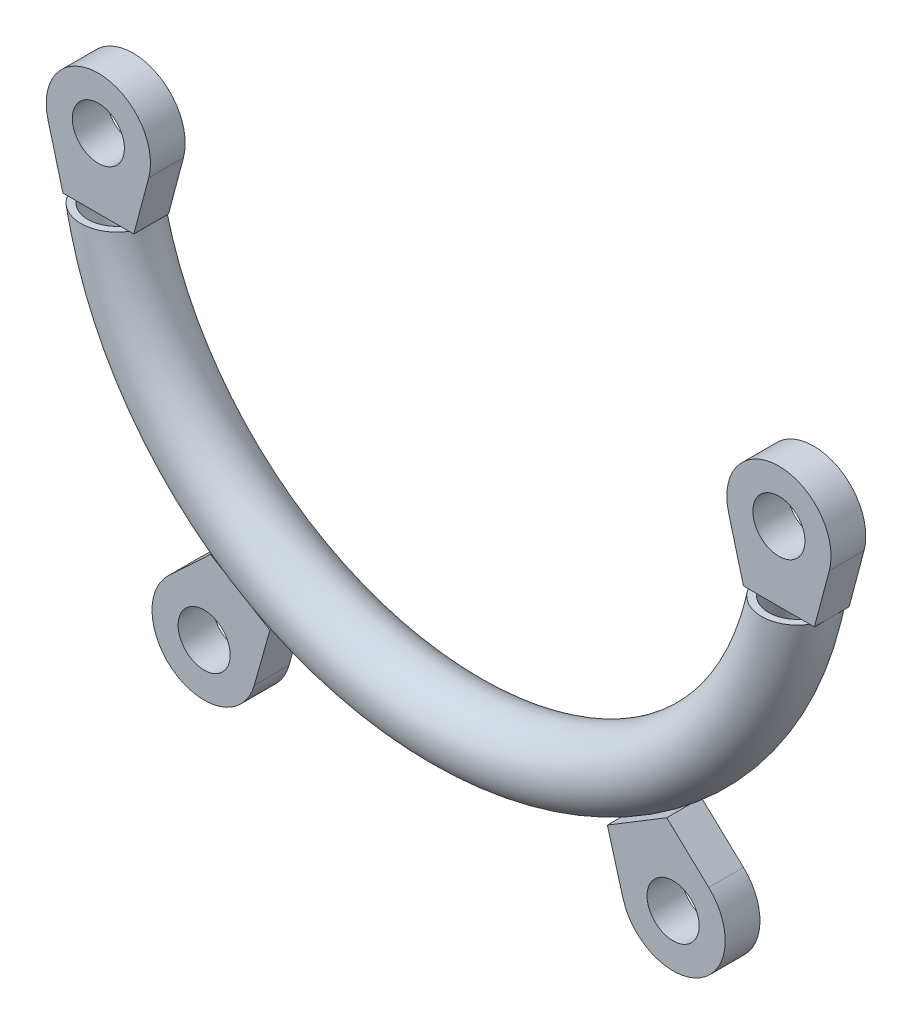
from build123d import *

# Parameters (mm, degrees)
SKETCH_2_R               = 10
SKETCH_2_R_2             = 8
CUT_EXTRUDE_1_DEPTH      = 156.884572829
CUT_EXTRUDE_1_DEPTH_BACK = 156.884572829
SKETCH_4_R               = 7.5
EXTRUDE_1_DEPTH          = 5
SKETCH_5_R               = 7.5
EXTRUDE_2_DEPTH          = 5
EXTRUDE_2_2_DEPTH        = 5


with BuildPart() as part:
    # 扫描1: sweep along a path in 草图1
    with BuildLine(Plane.XY) as sweep_1_path:
        CenterArc((0, 0), 100, 0, 360)
    # 草图2 → 扫描1 (sweep)
    with BuildSketch(Plane(origin=(0, 0, 0), x_dir=(0, 0, -1), z_dir=(1, 0, 0))):
        with Locations((0, -100)):
            Circle(SKETCH_2_R)
        with Locations((0, -100)):
            Circle(SKETCH_2_R_2, mode=Mode.SUBTRACT)
    sweep(path=sweep_1_path.line)

    # 草图3 → 切除-拉伸1 (cut, two sides: drawn at the far end of the back side and taken through both)
    with BuildSketch(Plane.XY.offset(-CUT_EXTRUDE_1_DEPTH_BACK)):
        Polygon((-124.821104754, -20), (0, -20), (127.823184446, -20), (127.823184446, 142.660997567), (-124.821104754, 142.660997567), align=None)
    extrude(amount=CUT_EXTRUDE_1_DEPTH + CUT_EXTRUDE_1_DEPTH_BACK, mode=Mode.SUBTRACT)

    # 草图4 → 凸台-拉伸1 (add, symmetric)
    with BuildSketch(Plane.XY):
        with BuildLine():
            Line((-108.166537158, -20.000005979), (-112.455542967, -3.850181648))
            ThreePointArc((-112.455542967, -3.850181648), (-97.958089835, 14.999994021), (-83.460636703, -3.850181648))
            Line((-83.460636703, -3.850181648), (-87.749642511, -20.000005979))
            Line((-87.749642511, -20.000005979), (-108.166537158, -20.000005979))
        make_face()
        with Locations((-97.958089835, -5.979e-06)):
            Circle(SKETCH_4_R, mode=Mode.SUBTRACT)
    extrude_1 = extrude(amount=EXTRUDE_1_DEPTH, both=True)

    # 镜向1: 凸台-拉伸1 across plane
    add(extrude_1.mirror(Plane(origin=(0, 0, 0), x_dir=(0, 0, 1), z_dir=(1, 0, 0))))


with BuildPart() as body_2:
    # 草图5 → 凸台-拉伸2 (new, symmetric)
    with BuildSketch(Plane.XY):
        with BuildLine():
            Line((-65.661725401, -88.817440952), (-48.56904383, -99.202056337))
            Line((-48.56904383, -99.202056337), (-53.06070847, -115.165293752))
            ThreePointArc((-53.06070847, -115.165293752), (-75.288461538, -123.921941395), (-77.759418607, -100.159654982))
            Line((-77.759418607, -100.159654982), (-65.661725401, -88.817440952))
        make_face()
        with Locations((-67.5, -111.102430216)):
            Circle(SKETCH_5_R, mode=Mode.SUBTRACT)
    extrude(amount=EXTRUDE_2_DEPTH, both=True)


with BuildPart() as body_3:
    # 草图5 → Extrude 2 2 (new, symmetric)
    with BuildSketch(Plane.XY):
        with BuildLine():
            Line((65.661725401, -88.817440952), (77.759418607, -100.159654982))
            ThreePointArc((77.759418607, -100.159654982), (75.288461538, -123.921941395), (53.06070847, -115.165293752))
            Line((53.06070847, -115.165293752), (48.56904383, -99.202056337))
            Line((48.56904383, -99.202056337), (65.661725401, -88.817440952))
        make_face()
        with Locations(Location((67.5, -111.102430216, 0), (0, 0, 180))):
            Circle(SKETCH_5_R, mode=Mode.SUBTRACT)
    extrude(amount=EXTRUDE_2_2_DEPTH, both=True)


solid = Compound([part.part, body_2.part, body_3.part])
